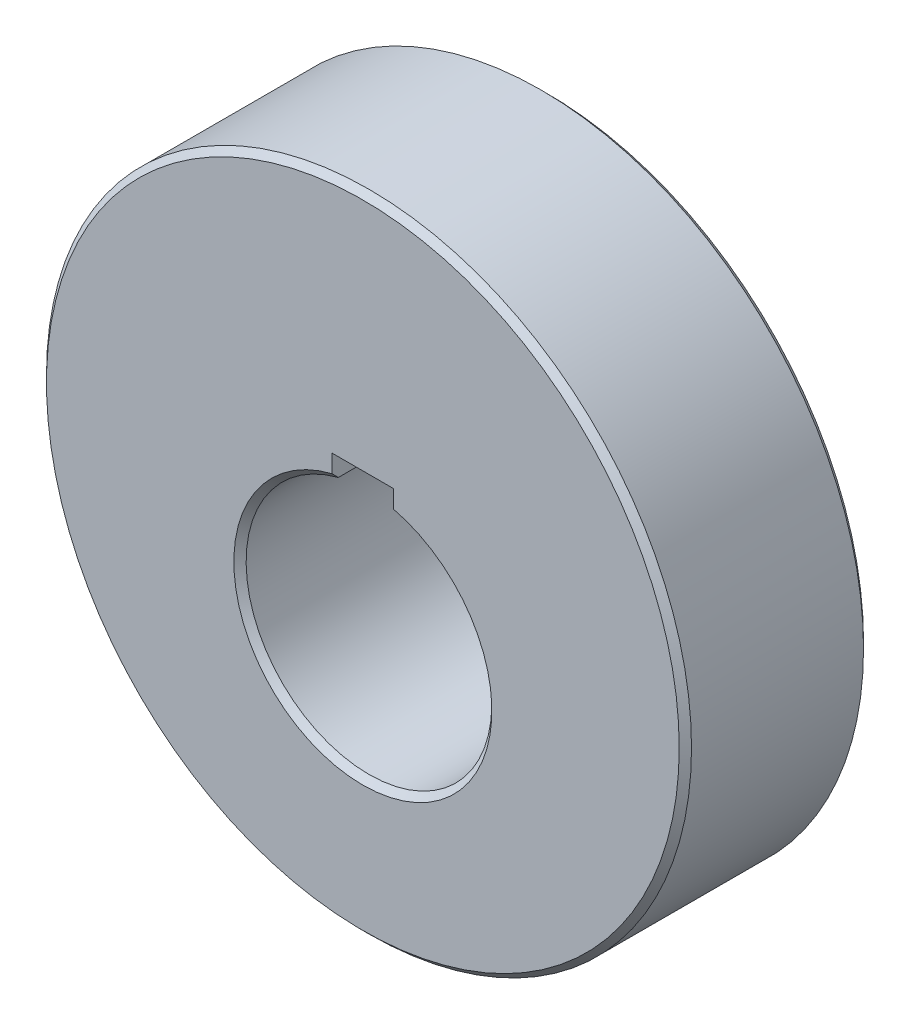
from build123d import *

# Parameters (mm, degrees)
SKETCH_1_4_R       = 52.5
EXTRUDE1_DEPTH     = 30
SKETCH_1_3_R       = 30
EXTRUDE2_DEPTH     = 18
CUT_EXTRUDE1_DEPTH = 87.962635655
CHAMFER1_SIZE      = 1


with BuildPart() as part:
    # Sketch 1_4 → Extrude1 (new body)
    with BuildSketch(Plane.XY):
        with Locations((0, 10)):
            Circle(SKETCH_1_4_R)
    extrude(amount=EXTRUDE1_DEPTH)

    # 草图1<3> → Extrude2 (add)
    with BuildSketch(Plane.XY):
        Circle(SKETCH_1_3_R)
        with BuildLine():
            Line((5, 19.364916731), (5, 23.3))
            Line((5, 23.3), (-5, 23.3))
            Line((-5, 23.3), (-5, 19.364916731))
            ThreePointArc((-5, 19.364916731), (0, -20), (5, 19.364916731))
        make_face(mode=Mode.SUBTRACT)
    extrude(amount=-EXTRUDE2_DEPTH)

    # Sketch 1_4 2 → Cut-Extrude1 (cut, through all)
    with BuildSketch(Plane.XY):
        with BuildLine():
            Line((5, 19.364916731), (5, 23.3))
            Line((5, 23.3), (-5, 23.3))
            Line((-5, 23.3), (-5, 19.364916731))
            ThreePointArc((-5, 19.364916731), (0, -20), (5, 19.364916731))
        make_face()
    extrude(amount=CUT_EXTRUDE1_DEPTH, mode=Mode.SUBTRACT)

    # Chamfer1
    chamfer1_edges = [part.edges().sort_by_distance(p)[0] for p in [
        (-52.5, 10, 0),
        (0, -20, 30),
        (-52.5, 10, 30),
        (-30, 0, -18),
        (0, -20, -18),
    ]]
    chamfer(chamfer1_edges, length=CHAMFER1_SIZE)


solid = part.part
